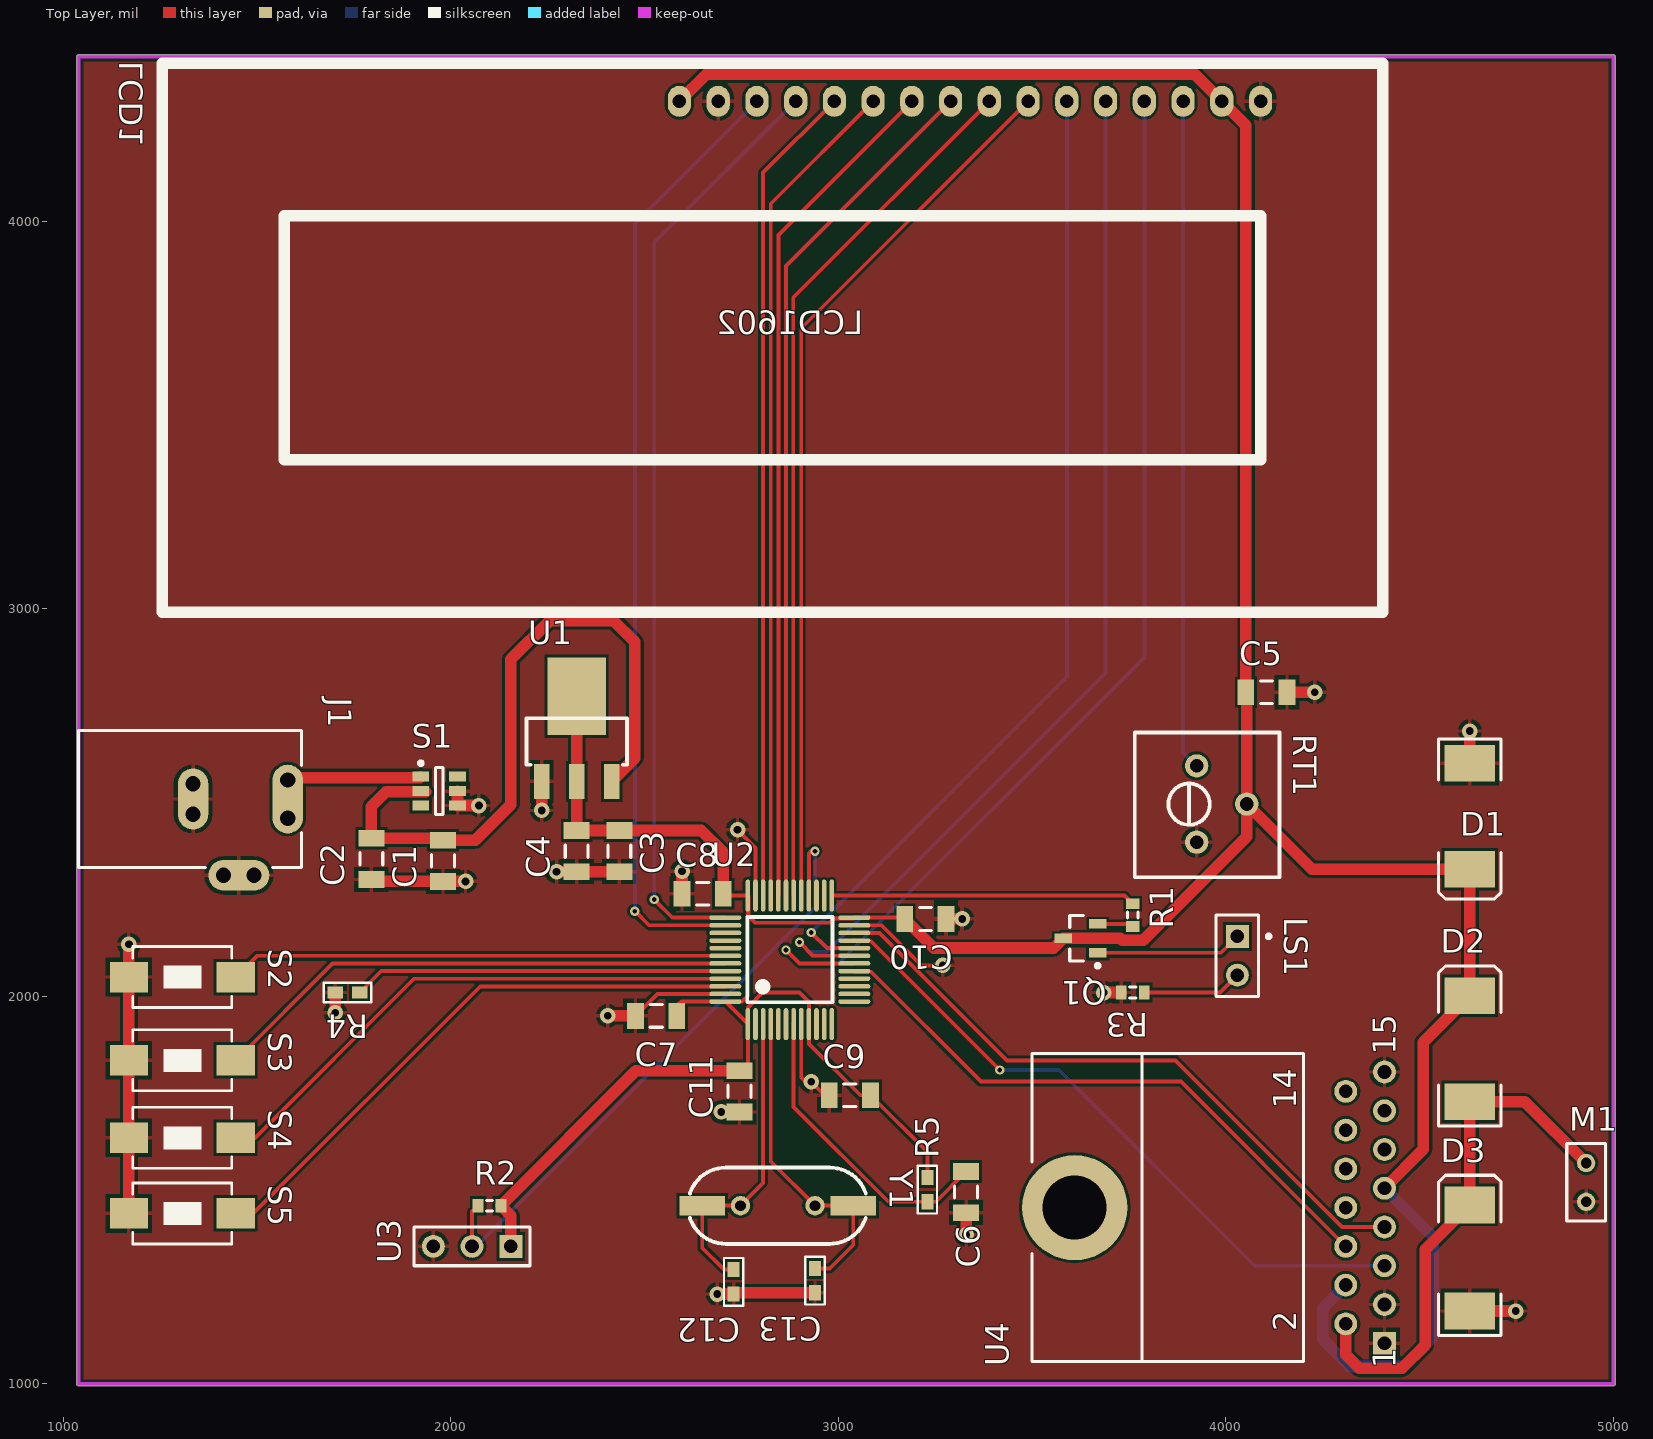
[diagram p0: Top Layer view]
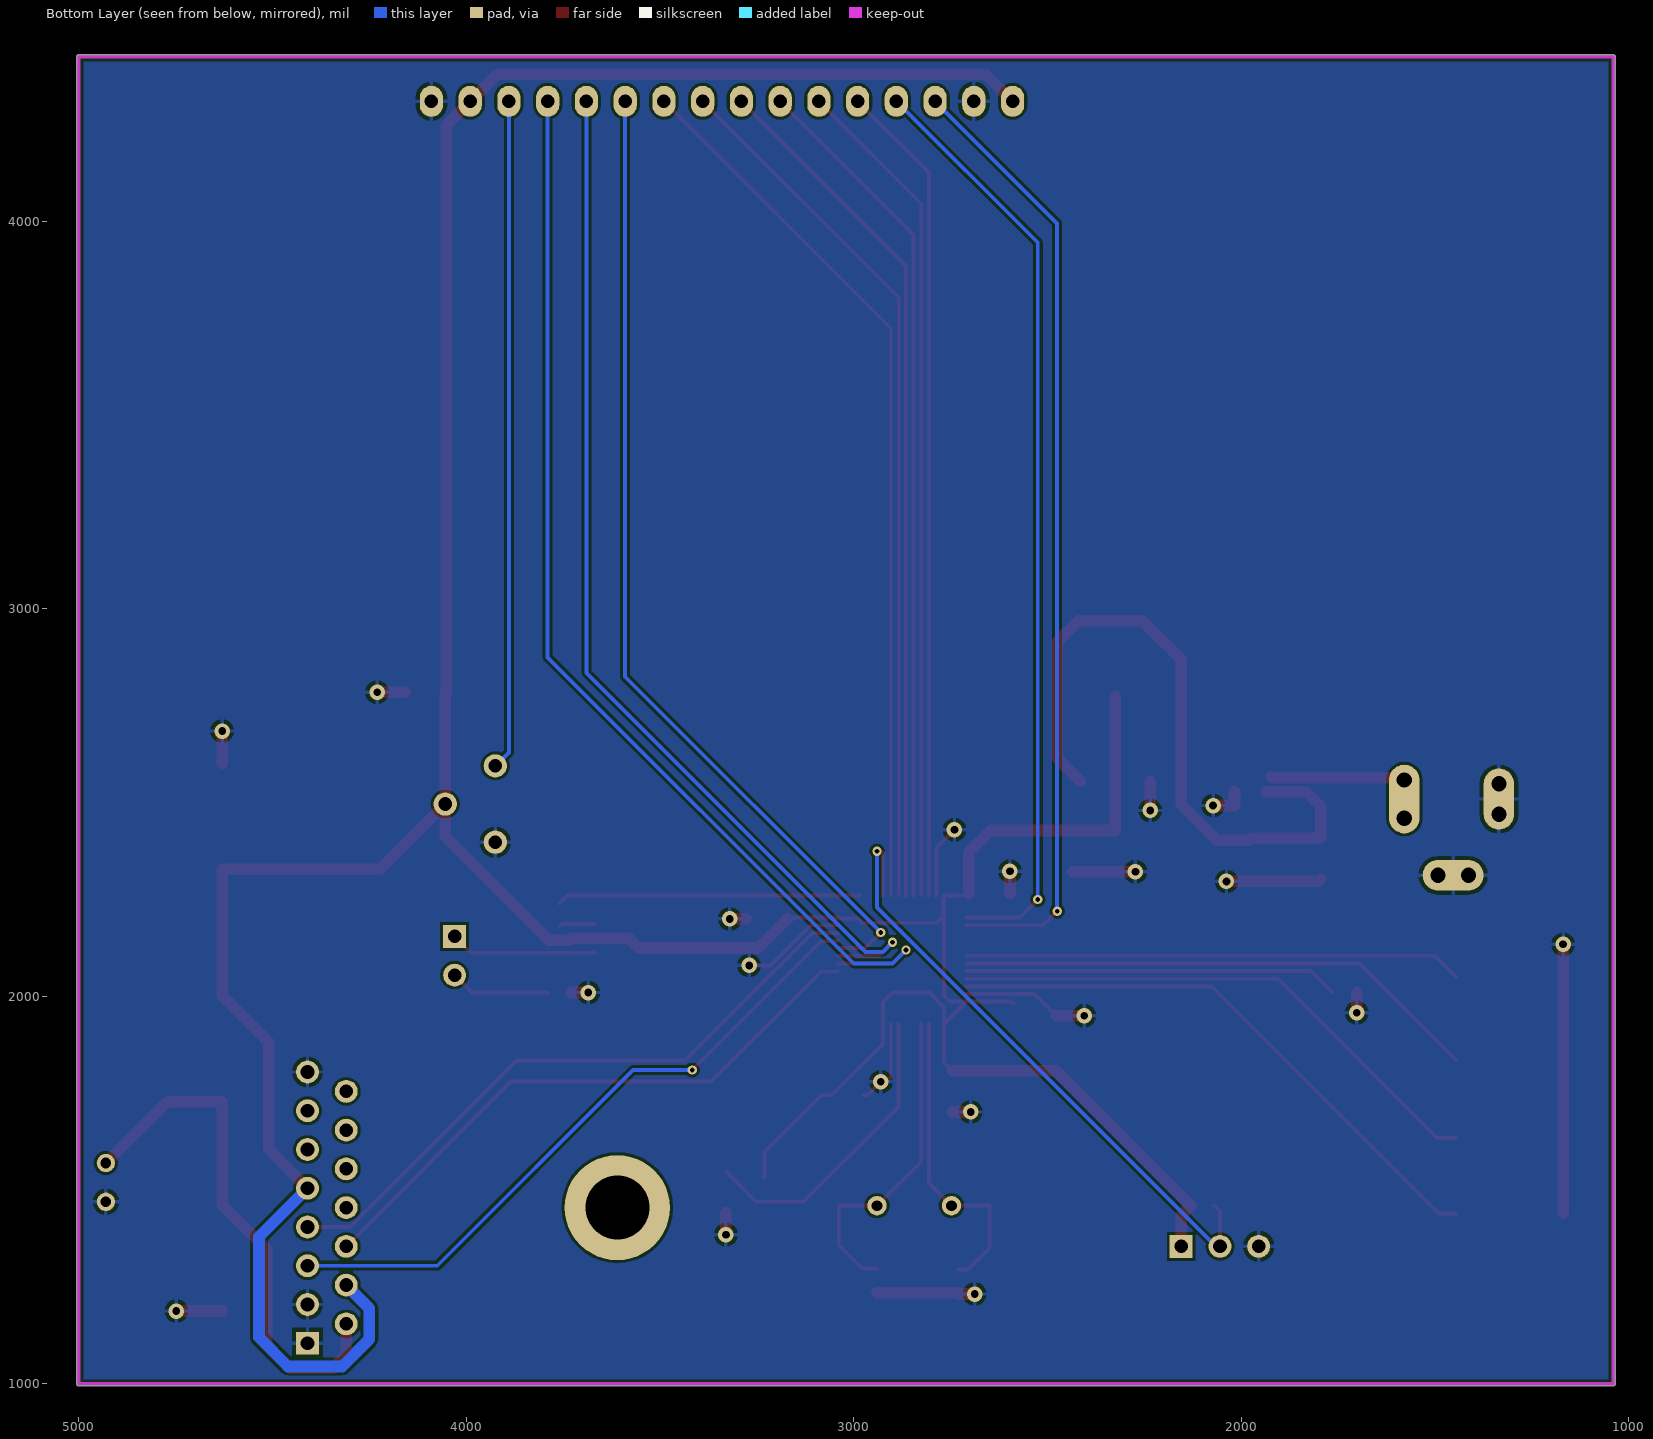
[diagram p1: Bottom Layer view, seen from below]
# Altium PCB MISC82673.PcbDoc
Units mil, origin at the board's own origin, x right, y up, seen from the top; angles counter-clockwise.
Board outline 3970.03 x 3435.03 mil, 2 copper layers (Top Layer, Bottom Layer); 37 components, 33 nets, 166 pads, 26 vias.

## Layer stack, top to bottom (the 12.6 mil dielectric is the usual default, probably not edited)
Top Solder: solder mask 0.4, Solder Resist, Dk 3.5
Top Layer: signal copper 1.4
Dielectric 1: dielectric 12.6, FR-4, Dk 4.8
Bottom Layer: signal copper 1.4
Bottom Solder: solder mask 0.4, Solder Resist, Dk 3.5

## Board outline
1034.98,1000 ccw(c1040,1000) 1040,994.99 5000,994.99 ccw(c5000,1000) 5005.02,1000 5005.02,4425 ccw(c5000,4425) 5000,4430.02 1040,4430.02 ccw(c1040,4425) 1034.98,4425

## Design rules (kind name [scope] priority, off if disabled: settings)
Clearance [All] p1: gap=7 except(0: Arc-Text Track-Text SMDPad-Text THPad-Text Via-Text Fill-Text Poly-Text Region-Text Text-Text)
MinimumSolderMaskSliver [All] p1: minsoldermaskwidth=0
PolygonConnect [All] p1: connectstyle=Relief reliefconductorwidth=10 reliefentries=4 polygonreliefangle="90 Angle" airgapwidth=10
RoutingVias [All] p1: holewidth=28 width=50 viastyle="Through Hole" minholewidth=28 minwidth=50 maxholewidth=28 maxwidth=50
SilkToSilkClearance [All] p1: silktosilkclearance=0
SilkToSolderMaskClearance [IsPad] p1: minsilkscreentomaskgap=0 clearancetoexposedcopper=TRUE
SolderMaskExpansion [All] p1: expansion=4
Width [All] p1: maxlimit=30 minlimit=10 preferedwidth=10
27 further rules are at their usual default settings.

## Components (designator, comment, footprint, x,y, rotation, side; value= is the part's Value field where it differs from the comment)
C1 "100PF" C1206 1980,2350 r90 top
C2 "100PF" C1206 1795,2355 r90 top
C3 "100PF" C1206 2435,2375 r90 top
C4 "100PF" C1206 2325,2375 r90 top
C5 "1U" C1206 4105,2785 r0 top
C6 "0.1UF" C1206 3330,1495 r90 top
C7 "0.1UF" C1206 2530,1950 r0 top
C8 "0.1UF" C1206 2650,2265 r0 top
C9 "0.1UF" C1206 3030,1745 r0 top
C10 "0.1UF" C1206 3225,2200 r180 top
C11 "0.1UF" C1206 2745,1755 r90 top
C12 "22P" my0603 2730,1295 r270 top
C13 "22P" my0603 2940,1297.99 r270 top
D1 "Diode" SMC 4630,2465 r270 top
D2 "Diode" SMC 4630,1865 r90 top
D3 "Diode" SMC 4630,1325 r90 top
J1 "PWR2.5" KLD-0202 1039.72,2509.37 r0 top
LCD1 "LCD1602" LCD1602 4090,4310 r180 top
LS1 "Speaker" PIN2 4030,2155 r270 top
M1 "Meter" RAD-0.1 4930,1520 r90 top
Q1 "PNP" SOT-23B_N 3625,2150 r180 top
R1 "100" J1-0603 3760,2210 r90 top
R2 "10K" J1-0603 2100,1460 r0 top
R3 "100" J1-0603 3760,2010 r180 top
R4 "Res2" my0603 1765,2010 r180 top
R5 "Res2" my0603 3230,1470 r90 top
RT1 "10K" 电位器 3940.12,2494.56 r270 top
S1 "SW DPDT" SOT23-6_N 1970,2530 r0 top
S2 "SW-PB" SW_PB2_A1 1305,2050 r270 top
S3 "SW-PB" SW_PB2_A1 1305,1835 r270 top
S4 "SW-PB" SW_PB2_A1 1305,1635 r270 top
S5 "SW-PB" SW_PB2_A1 1305,1440 r270 top
U1 "AMS1117" SOT223 2325,2555 r0 top
U2 "STM32F103C8T6" "LQFP48 7X7" 2875,2095 r0 top
U3 "DS18B20" HDR1X3 2155,1355 r180 top
U4 "L298N" Multiwatt15H 4010,1455 r90 top
Y1 "12M" XTAL_US 2747.87,1460 r0 top

## Footprints (in the part's own frame and the unit in brackets; to place one, negate y for a bottom-side part, rotate by r counter-clockwise, add the part's x,y. Pads: shape width x height; smd on the part's side, far side on the other; paste and mask are expansions set on the pad)
C1206 [mm] "Chip Capacitor, Body 3.2x1.6mm, IPC High Density"
  rect 1.1x1.7 smd: 1(-1.35,0) 2(1.35,0)
  silkscreen extent -0.4,-0.75 0.4,0.75, body extent -1.7,-0.9 1.7,0.9, height 1.3
HDR1X3 [mm] "Connector; Header; 3 Position"
  rect 1.5x1.5 hole 0.9: 1(0,0)
  round 1.5 hole 0.9: 2(2.54,0) 3(5.08,0)
  silkscreen extent -1.27,-1.27 6.35,1.27
J1-0603 [mm] "Chip Resistor, Body 1.6x0.8mm, IPC High Density"
  rect 0.7x0.9 smd: 1(-0.75,0) 2(0.75,0)
  silkscreen extent -0.2,-0.35 0.2,0.35, body extent -0.85,-0.48 0.85,0.48, height 0.9
KLD-0202 [mm] "DC Power Jack, 2.5mm, KLD Series, PCB Mount"
  oval 2x4.5 all layers, no hole: 1(13.7,0)
  round 1.5 hole 1: 1A(13.7,-1.25) 1B(13.7,1.25) 2A(7.5,-1) 2B(7.5,1) 3A(9.5,-5) 3B(11.5,-5)
  oval 2x4 all layers, no hole: 2(7.5,0)
  oval 4x2 all layers, no hole: 3(10.5,-5)
  silkscreen extent 0,-4.5 14.6,4.5
LCD1602 [mil]
  oval 60x80 hole 35.43: 1(0,0) 2(100,0) 3(200,0) 4(300,0) 5(400,0) 6(500,0) 7(600,0) 8(700,0) 9(800,0) 10(900,0) 11(1000,0) 12(1100,0) 13(1200,0) 14(1300,0) 15(1400,0) 16(1500,0)
  silkscreen extent -315,-98 2835,1319, body extent -315,-80 2854,1357, height 414
"LQFP48 7X7" [mm]
  oval 0.3x2.1 smd: 1(-2.75,-4.227) 2(-2.25,-4.227) 3(-1.75,-4.227) 4(-1.25,-4.227) 5(-0.75,-4.227) 6(-0.25,-4.227) 7(0.25,-4.227) 8(0.75,-4.227) 9(1.25,-4.227) 10(1.75,-4.227) 11(2.25,-4.227) 12(2.75,-4.227) 25(2.75,4.202) 26(2.25,4.202) 27(1.75,4.202) 28(1.25,4.202) 29(0.75,4.202) 30(0.25,4.202) 31(-0.25,4.202) 32(-0.75,4.202) 33(-1.25,4.202) 34(-1.75,4.202) 35(-2.25,4.202) 36(-2.75,4.202)
  oval 2.1x0.3 smd: 13(4.227,-2.75) 14(4.227,-2.25) 15(4.227,-1.75) 16(4.227,-1.25) 17(4.227,-0.75) 18(4.227,-0.25) 19(4.227,0.25) 20(4.227,0.75) 21(4.227,1.25) 22(4.227,1.75) 23(4.227,2.25) 24(4.227,2.75) 37(-4.227,2.75) 38(-4.227,2.25) 39(-4.227,1.75) 40(-4.227,1.25) 41(-4.227,0.75) 42(-4.227,0.25) 43(-4.227,-0.25) 44(-4.227,-0.75) 45(-4.227,-1.25) 46(-4.227,-1.75) 47(-4.227,-2.25) 48(-4.227,-2.75)
  silkscreen extent -2.79,-2.79 2.79,2.79, body extent -4.51,-4.5 4.5,4.5, height 1.45
Multiwatt15H [mm] "TO, Thru-Hole, Horizontal, Heatsink Mounted; 15 Bent Staggered Leads; Pitch 1.27 mm"
  rect 1.5x1.5 hole 0.9: 1(-8.89,-10.155)
  round 1.5 hole 0.9: 2(-7.62,-7.615) 3(-6.35,-10.155) 4(-5.08,-7.615) 5(-3.81,-10.155) 6(-2.54,-7.615) 7(-1.27,-10.155) 8(0,-7.615) 9(1.27,-10.155) 10(2.54,-7.615) 11(3.81,-10.155) 12(5.08,-7.615) 13(6.35,-10.155) 14(7.62,-7.615) 15(8.89,-10.155)
  round 6.9 hole 4.2: 16(0,10.155)
  silkscreen extent -10.1,-4.84 10.1,12.96
my0603 [mm]
  rect 1x0.8 smd: 1(0,0) 2(1.6,0)
  silkscreen extent -0.76,-0.64 2.36,0.64
PIN2 [mm] "Photosensitive Diode; 2 Leads"
  rect 1.5x1.5 hole 0.9: 1(0,0)
  round 1.5 hole 0.9: 2(2.54,0)
  silkscreen extent -1.4,-1.4 3.94,2.18
RAD-0.1 [mm] "Radial Cap, Thru-Hole; 2 Leads; 0.1 in Pin Spacing"
  round 1.2 hole 0.7: 1(-1.27,0) 2(1.27,0)
  silkscreen extent -2.54,-1.27 2.54,1.27
SMC [mm] "DO-214-AB/SMC; 2 C-Bend Leads; Body 7.9 x 5.9 mm, inc. leads (LxW)"
  rect 2.4x3.3 smd: 1(-3.475,0) 2(3.475,0)
  silkscreen extent -5.07,-2.05 5.43,2.05
SOT23-6_N [mm] "SOT23, 6-Leads, Body 2.9x1.6mm, Pitch 0.95mm, Lead Span 2.7mm, IPC Medium Density"
  rect 1.1x0.65 smd: 1(-1.2,0.95) 2(-1.2,0) 3(-1.2,-0.95) 4(1.2,-0.95) 5(1.2,0) 6(1.2,0.95)
  silkscreen extent -1.32,-1.55 0.25,1.95, body extent -0.9,-1.55 0.9,1.55, height 1.45
SOT223 [mil]
  rect 40x90 smd: 1(-90,0) 2(0,0) 3(90,0)
  rect 150x200 smd: 2(0,220)
  silkscreen extent -130,43 130,163, body extent -130,-30 126,246, height 65
SOT-23B_N [mm] "SOT23, 3-Leads, Body 2.9x1.3mm, Pitch 0.95mm, Lead Span 2.4mm, IPC Medium Density"
  rect 1.15x0.6 smd: 1(-1.125,0.95) 2(-1.125,-0.95) 3(1.125,0)
  silkscreen extent -1.25,-1.5 0.7,1.92, body extent -0.7,-1.5 0.7,1.5, height 1.14
SW_PB2_A1 [mm]
  rect 2x2.5 smd: 1(0,3.556) 2(0,-3.444)
  silkscreen extent -2,-3.19 2,3.31, body extent -2.03,-3.18 2.03,3.3, height 1.2
XTAL_US [mm]
  rect 3x1.27 smd: 1(-2.51,0) 2(7.39,0)
  round 1.27 hole 0.711: 1(0,0) 2(4.88,0)
  silkscreen extent -3.33,-2.5 8.21,2.5
电位器 [mil]
  round 60 hole 35.43 paste+0 mask+2: 1(96.41,-15.12) 2(-2.01,114.1) 3(-100.44,-15.12)
  silkscreen extent -187,-175 187,199

## Part data
C1 C2 C3 C4 C5 C6 C7 C8 C9 C10 C11: library part "Cap Semi", "Capacitor (Semiconductor SIM Model)"
C12 C13: library part CAP, "Capacitor"
D1 D2 D3: "Default Diode"
J1: "Low Voltage Power Supply Connector"
LS1: "Loudspeaker"
M1: "Indicating Instrument"
Q1: "PNP Bipolar Transistor"
R1 R2 R3: library part Res3, "Resistor"
R4 R5: "Resistor"
RT1: library part 电位器
S1 S2 S3 S4 S5: "Switch"
U1: "Three-terminal voltage regulator"
U4: "Dual Full Bridge Driver"
Y1: library part XTAL, "Crystal Oscillator"

## Via types
v1: diameter 40, hole 20, Top Layer to Bottom Layer, 19 vias
v2: diameter 24, hole 12, Top Layer to Bottom Layer, 7 vias

## Nets (pads, with @x,y where several pads share a name; then routed paths per layer and width w, separated by ;. In a path a pad name is that pad's centre, name@x,y a point inside that pad or via, vN(x,y) a via of type N, cw(c..) or ccw(c..) an arc to the next point about the centre after c; other vN are vias at no path point)
+5: C1.2 C2.2 S1.2 U1.3 | length 1782.2
  Top Layer w30: S1.2@1935.48,2527.8 1832.8,2527.8 1795,2490 C2.2 1975,2408.15 C1.2 2063.15,2403.15 2155,2495 2155,2870 2255,2970 2420,2970 2475,2915 2475,2615 U1.3
GND: C1.1 C2.1 C3.1 C4.1 C5.2 C6.1 C7.1 C8.1 C9.1 C10.1 C11.1 C12.2 C13.2 D1.1 D3.1 J1.2 J1.2A J1.2B J1.3 J1.3A J1.3B LCD1.1 LCD1.15 M1.1 R3.2 R4.2 RT1.1 S1.4 S1.5 S2.2 S3.2 S4.2 S5.2 U1.1 U2.8 U2.23 U2.35 U2.47 U3.3 U4.1 U4.3 U4.15 | length 3113.4
  Top Layer w10: C7.1 2533.27,2006.42 U2.47 ; v1(2740,2430) 2786.42,2383.58 U2.35 ; U2.8 2904.53,1790.47 2915,1780 v1(2930,1780) 2965,1745 C9.1 ; U2.23 3111.42,2183.58 3215,2080 v1(3270,2080)
  Top Layer w30: S5.2 S4.2 S3.2 S2.2 v1(1169.41,2134.41) ; v1(1702.01,1957.99) R4.2 ; C2.1 1800,2296.85 C1.1 v1(2038.15,2296.85) ; S1.5 S1.4 v1(2072.6,2492.6) ; v1(2235,2480) U1.1 ; v1(2273.15,2321.85) C4.1 C3.1 ; v1(2405,1950) C7.1 ; C8.1 v1(2596.85,2323.15) ; v1(2687.99,1232.01) C12.2 2732.99,1235 C13.2 ; v1(2698.15,1701.85) C11.1 ; C10.1 v1(3320,2200) ; v1(3330,1385) C6.1 ; v1(3685,2010) R3.2 ; C5.2 v1(4230,2785) ; D3.1 v1(4748.19,1188.19) ; D1.1 v1(4630,2685)
NetC6_2: C6.2 R5.1 U2.7 | length 792.6
  Top Layer w10: U2.7 2884.84,1715 3129.84,1470 R5.1 3251.85,1470 C6.2
NetD2_1: D2.1 D3.2 M1.2 U4.2 | length 1365.8
  Top Layer w30: U4.2 4309.8,1075.2 4345,1040 4455,1040 4515,1100 4515,1346.81 D3.2 D2.1 4771.81,1728.19 M1.2
NetJ1_1: J1.1 J1.1A J1.1B S1.1 | length 351
  Top Layer w30: J1.1B 1579.09,2564.8 1920.15,2564.8 S1.1
NetLCD1_3: LCD1.3 RT1.3 | length 1729.5
  Bottom Layer w10: LCD1.3 3890,2630 RT1.3
NetLS1_1: LS1.1 Q1.1 | length 378.3
  Top Layer w10: Q1.1 3987.6,2112.6 LS1.1
NetLS1_2: LS1.2 R3.1 | length 259.1
  Top Layer w10: R3.1 3985,2010 LS1.2
NetQ1_2: Q1.2 R1.1 | length 93.6
  Top Layer w10: Q1.2 3753.07,2187.4 R1.1
NetR4_1: R4.1 U2.44 | length 966.6
  Top Layer w10: R4.1 1820.47,2065.47 U2.44
OSC_IN: C12.1 U2.3 Y1.1 | length 804.7
  Top Layer w10: C12.1 2705,1295 2649.06,1350.94 2649.06,1460 2747.87,1460 2806.1,1518.23 U2.3
OSC_OUT: C13.1 U2.4 Y1.2 | length 839.9
  Top Layer w10: U2.4 2825.79,1574.21 2940,1460 3038.82,1460 3038.82,1358.82 2977.99,1297.99 C13.1
PA7: U2.17 U4.6 | length 1562.7
  Top Layer w10: U2.17 3043.2,2063.69 3084.27,2063.69 3367.96,1780 3884.8,1780 U4.6
PA8: LCD1.7 U2.29 | length 2292.1
  Top Layer w10: U2.29 2904.53,3724.53 LCD1.7
PA9: LCD1.8 U2.30 | length 2259.5
  Top Layer w10: U2.30 2884,2261.26 2884,3804 LCD1.8
PA10: LCD1.9 U2.31 | length 2225.6
  Top Layer w10: U2.31 2865.16,3885.16 LCD1.9
PA11: LCD1.10 U2.32 | length 2192.3
  Top Layer w10: U2.32 2845.47,3965.47 LCD1.10
PA12: LCD1.11 U2.33 | length 2159
  Top Layer w10: U2.33 2825.79,4045.79 LCD1.11
PA13: LCD1.12 U2.34 | length 2125.8
  Top Layer w10: U2.34 2806.1,4126.1 LCD1.12
PA14: LCD1.13 U2.37 | length 2414.1
  Top Layer w10: v2(2525,2250) 2571.73,2203.27 U2.37
  Bottom Layer w10: v2(2525,2250) 2525,3945 LCD1.13
PA15: LCD1.14 U2.38 | length 2469.1
  Top Layer w10: v2(2475,2220) 2511.42,2183.58 U2.38
  Bottom Layer w10: v2(2475,2220) 2475,3995 LCD1.14
PB0: LCD1.4 U2.18 | length 2892.6
  Top Layer w10: v2(2865,2120) 2899.84,2085.16 U2.18
  Bottom Layer w10: v2(2865,2120) 2900,2085 3000,2085 3790,2875 LCD1.4
PB1: LCD1.5 U2.19 | length 2729.6
  Top Layer w10: v2(2900,2140) 2935.16,2104.84 U2.19
  Bottom Layer w10: v2(2900,2140) 2925,2115 2970,2115 3690,2835 LCD1.5
PB2: LCD1.6 U2.20 | length 2546.6
  Top Layer w10: v2(2930,2165) 2970.47,2124.53 U2.20
  Bottom Layer w10: v2(2930,2165) 3590,2825 LCD1.6
PB6: S2.1 U2.42 | length 1286.3
  Top Layer w10: S2.1 1499.84,2104.84 U2.42
PB7: S3.1 U2.43 | length 1367.2
  Top Layer w10: S3.1 1695.16,2085.16 U2.43
PB8: S4.1 U2.45 | length 1433.7
  Top Layer w10: S4.1 1495,1635 1905.79,2045.79 U2.45
PB9: S5.1 U2.46 | length 1506.4
  Top Layer w10: S5.1 1490,1440 2076.1,2026.1 U2.46
PB10: U2.21 U4.5 | length 1716
  Top Layer w10: U2.21 3043.2,2142.43 3084.27,2142.43 v2(3416.7,1810)
  Bottom Layer w10: v2(3416.7,1810) 3570,1810 4075,1305 U4.5
PB11: U2.22 U4.7 | length 1682.7
  Top Layer w10: U2.22 3106.1,2163.9 3435,1835 3870,1835 4300,1405 U4.7
PB12: R1.2 U2.25 | length 785.4
  Top Layer w10: U2.25 3739.11,2260.42 R1.2
PB15: R2.1 U2.28 U3.2 | length 1630.8
  Top Layer w10: U3.2 2055,1444.53 R2.1 ; U2.28 2924.21,2369.21 2930,2375 v2(2940,2375)
  Bottom Layer w10: U3.2 2065,1355 2940,2230 v2(2940,2375)
VCC: C3.2 C4.2 C5.1 C7.2 C8.2 C9.2 C10.2 C11.2 D1.2 D2.2 LCD1.2 LCD1.16 Q1.3 R2.2 R5.2 RT1.2 U1.2 U2.1 U2.9 U2.24 U2.36 U2.48 U3.1 U4.4 U4.9 | length 10671.9
  Top Layer w10: C7.2@2588.15,1980 2594.88,1986.73 U2.48 ; C8.2 2707.73,2260.42 U2.36 ; C11.2 2766.73,1829.88 U2.1 ; C10.2 3155,2200 3151.73,2203.27 U2.24 3039.64,2201.49 2988.78,2201.49 2977.29,2190 2786.29,2190 2768.51,2207.78 2768.51,2258.64 U2.36 ; R5.2 3230,1598.15 C9.2 3056.94,1745 2924.21,1877.73 U2.9 2924.21,1985.79 2900,2010 2805,2010 2766.73,1971.73 U2.1 ; U2.48 2751.73,1986.73 2766.73,2001.73 U2.36 ; U2.48 U2.1
  Top Layer w30: U3.1 2155,1434.53 R2.2 2477.68,1808.15 C11.2 ; U1.2@2325,2775 2325,2555 C4.2 C3.2 2646.85,2428.15 2703.15,2371.85 C8.2 ; LCD1.16 2660,4380 3920,4380 LCD1.2 4051.85,4248.15 C5.1 4054.22,2782.63 RT1.2 ; C10.2 3246.85,2125 3555.71,2125 Q1.3 3727.86,2150 3733.17,2144.69 3786.83,2144.69 4054.22,2412.08 RT1.2 ; U4.9 4510,1605.2 4510,1881.81 D2.2 D1.2 4222.6,2328.19 RT1.2
  Bottom Layer w30: U4.4 4250,1195.2 4250,1115 4320,1045 4460,1045 4535,1120 4535,1379.8 U4.9
pads on no net: S1.3 S1.6 U2.2 U2.5 U2.6 U2.10 U2.11 U2.12 U2.13 U2.14 U2.15 U2.16 U2.26 U2.27 U2.39 U2.40 U2.41 U4.8 U4.10 U4.11 U4.12 U4.13 U4.14 U4.16

## Polygon pours and split planes (outlines as drawn)
GND on Top Layer "G" (solid, remove dead copper, pour order 0): 670,4585 820,4735 5230,4735 5230,780 5210,760 5105,865 750,865
GND on Bottom Layer "G" (solid, remove dead copper, pour order 2): 680,4620 5660,4620 5720,4560 5360,4200 5360,315 1000,315 635,680

## Keep-outs
Keep-Out Layer:
  lines w10: 1040,2320 1040,4425 1065,4425 ; 1040,2335 1040,1000 5000,1000 5000,4425 1050,4425